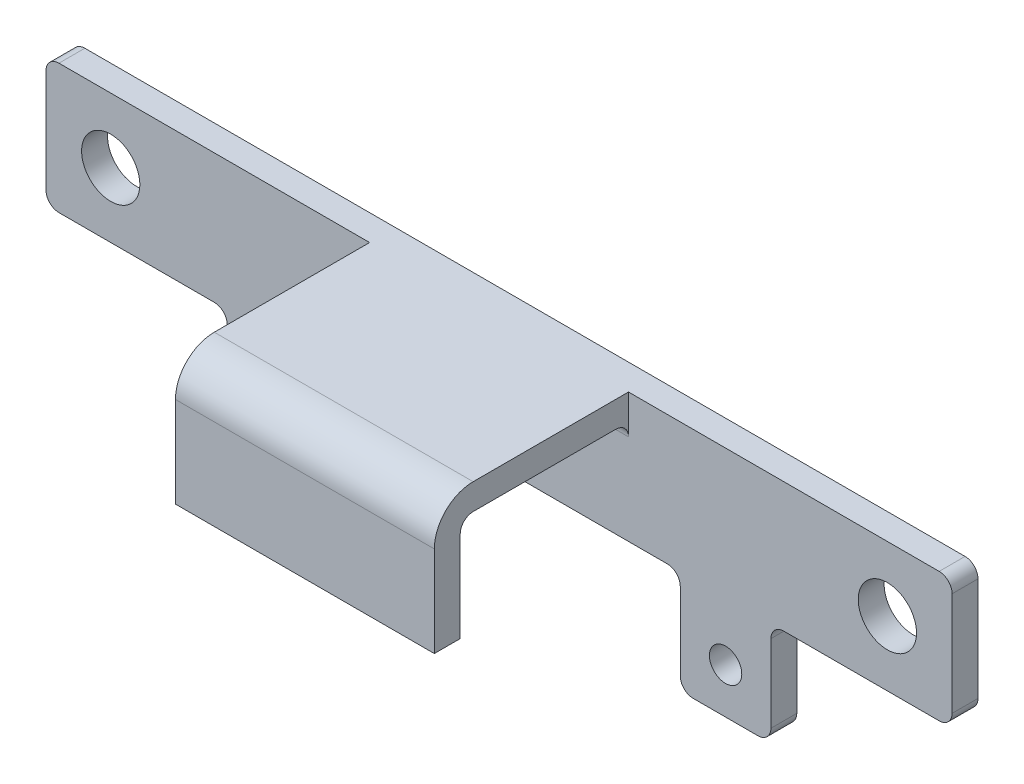
from build123d import *

# Parameters (mm, degrees)
SKETCH1_W             = 70
SKETCH1_H             = 10
BOSS_EXTRUDE1_DEPTH   = 2
SKETCH2_W             = 20
SKETCH2_H             = 2
BOSS_EXTRUDE2_DEPTH   = 15
SKETCH3_W             = 20
SKETCH3_H             = 2
BOSS_EXTRUDE3_DEPTH   = 8
FILLET2_R             = 1
FILLET3_R             = 3
SKETCH4_R             = 2.25
CUT_EXTRUDE1_DEPTH    = 8
SKETCH6_W             = 7
SKETCH6_H             = 2
BOSS_EXTRUDE4_DEPTH   = 8
FILLET4_R             = 1
M3_TAPPED_HOLE1_D     = 2.5
M3_TAPPED_HOLE1_DEPTH = 7.5
M3_TAPPED_HOLE1_TIP   = 0.751075774
FILLET5_R             = 1


with BuildPart() as part:
    # Sketch1 → Boss-Extrude1 (new body)
    with BuildSketch(Plane.XY):
        Rectangle(SKETCH1_W, SKETCH1_H)
    extrude(amount=BOSS_EXTRUDE1_DEPTH)

    # Sketch2 → Boss-Extrude2 (add)
    with BuildSketch(Plane.XY.offset(2)):
        with Locations((0, 4)):
            Rectangle(SKETCH2_W, SKETCH2_H)
    extrude(amount=BOSS_EXTRUDE2_DEPTH)

    # Sketch3 → Boss-Extrude3 (add)
    with BuildSketch(Plane(origin=(0, 3, 0), x_dir=(-1, 0, 0), z_dir=(0, -1, 0))):
        with Locations((0, -16)):
            Rectangle(SKETCH3_W, SKETCH3_H)
    extrude(amount=BOSS_EXTRUDE3_DEPTH)

    # Fillet2
    fillet2_edges = [part.edges().sort_by_distance(p)[0] for p in [
        (0, 3, 2),
        (0, 3, 15),
    ]]
    fillet(fillet2_edges, radius=FILLET2_R)

    # Fillet3
    fillet3_edges = [part.edges().sort_by_distance(p)[0] for p in [
        (0, 5, 17),
    ]]
    fillet(fillet3_edges, radius=FILLET3_R)

    # Sketch4 → Cut-Extrude1 (cut)
    with BuildSketch(Plane.XY.offset(2)):
        with Locations((-30, 0)):
            Circle(SKETCH4_R)
        with Locations((30, 0)):
            Circle(SKETCH4_R)
    extrude(amount=-CUT_EXTRUDE1_DEPTH, mode=Mode.SUBTRACT)

    # Sketch6 → Boss-Extrude4 (add)
    with BuildSketch(Plane(origin=(0, -5, 0), x_dir=(-1, 0, 0), z_dir=(0, -1, 0))):
        with Locations((-17.5, -1)):
            Rectangle(SKETCH6_W, SKETCH6_H)
        with Locations((17.5, -1)):
            Rectangle(SKETCH6_W, SKETCH6_H)
    extrude(amount=BOSS_EXTRUDE4_DEPTH)

    # Fillet4
    fillet4_edges = [part.edges().sort_by_distance(p)[0] for p in [
        (35, -5, 1),
        (-35, -5, 1),
        (-35, 5, 1),
        (35, 5, 1),
    ]]
    fillet(fillet4_edges, radius=FILLET4_R)

    # M3 Tapped Hole1
    with Locations(Plane(origin=(-17.5, -9.5, 2), x_dir=(1, 0, 0), z_dir=(0, 0, 1))):
        with Locations((0, 0), (35, 0)):
            Hole(M3_TAPPED_HOLE1_D / 2, depth=M3_TAPPED_HOLE1_DEPTH)
            with Locations((0, 0, -(M3_TAPPED_HOLE1_DEPTH + M3_TAPPED_HOLE1_TIP / 2))):  # 118° drill point
                Cone(0, M3_TAPPED_HOLE1_D / 2, M3_TAPPED_HOLE1_TIP, mode=Mode.SUBTRACT)

    # Fillet5
    fillet5_edges = [part.edges().sort_by_distance(p)[0] for p in [
        (14, -5, 1),
        (21, -5, 1),
        (14, -13, 1),
        (21, -13, 1),
        (-21, -5, 1),
        (-14, -5, 1),
        (-21, -13, 1),
        (-14, -13, 1),
    ]]
    fillet(fillet5_edges, radius=FILLET5_R)


solid = part.part
